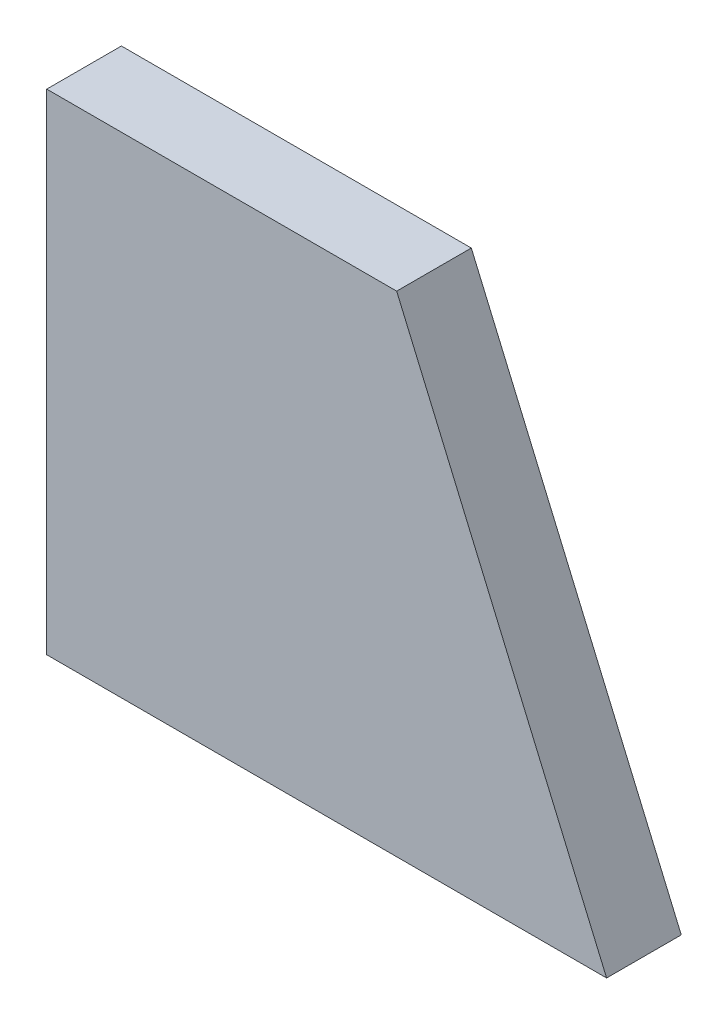
SolidWorks part; units mm, degrees
material "Q235B"
ref_plane "Front Plane" through (0, 0, 0) normal (0, 0, 1) x (1, 0, 0)
ref_plane "Top Plane" through (0, 0, 0) normal (0, 1, 0) x (1, 0, 0)
ref_plane "Right Plane" through (0, 0, 0) normal (1, 0, 0) x (0, 0, -1)
sketch "Sketch1" plane through (0, 0, 0) normal (0, 0, 1) x (1, 0, 0)
  line L0 (0, 0) -> (0, 105)
  line L1 (0, 105) -> (75, 105)
  line L2 (75, 105) -> (120, 0)
  line L3 (120, 0) -> (0, 0)
  dimension "D1" = 75
  dimension "D2" = 105
  dimension "D3" = 120
extrude "Boss-Extrude1" add sketch "Sketch1" along normal mid plane 16
sketch "Sketch2" plane through (0, 105, 0) normal (0, 1, 0) x (1, 0, 0)
  line L0 (0, 0) -> (-460, 0) construction
  circle A0 centre (-460, 0) radius 460 construction
  dimension "D1" = 920
